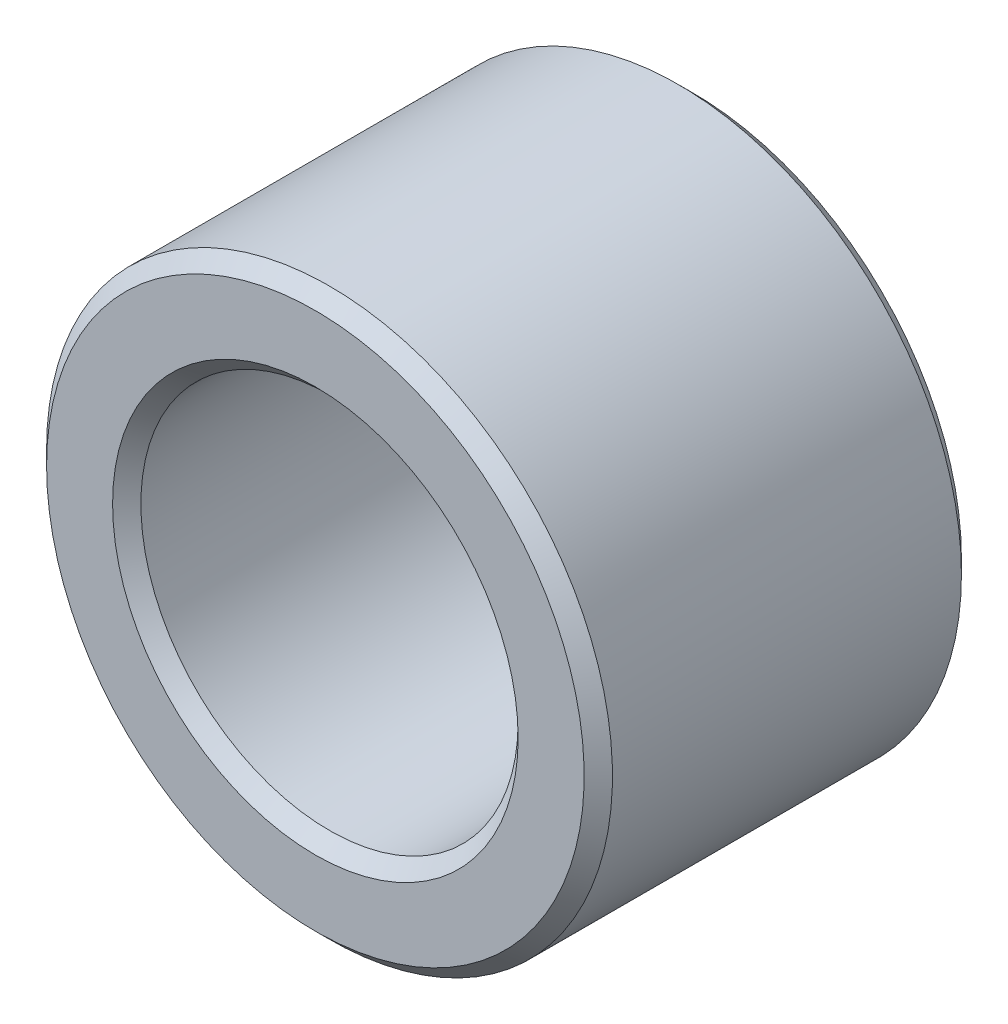
from build123d import *

# Parameters (mm, degrees)
SKETCH_1_R      = 6
SKETCH_1_R_2    = 4
EXTRUDE_1_DEPTH = 4
CHAMFER_1_SIZE  = 0.3


with BuildPart() as part:
    # 草图1 → 凸台-拉伸1 (new, symmetric)
    with BuildSketch(Plane.XY):
        Circle(SKETCH_1_R)
        Circle(SKETCH_1_R_2, mode=Mode.SUBTRACT)
    extrude(amount=EXTRUDE_1_DEPTH, both=True)

    # 倒角1
    chamfer_1_edges = [part.edges().sort_by_distance(p)[0] for p in [
        (-6, 0, -4),
        (-6, 0, 4),
        (-4, 0, -4),
        (-4, 0, 4),
    ]]
    chamfer(chamfer_1_edges, length=CHAMFER_1_SIZE)


solid = part.part
